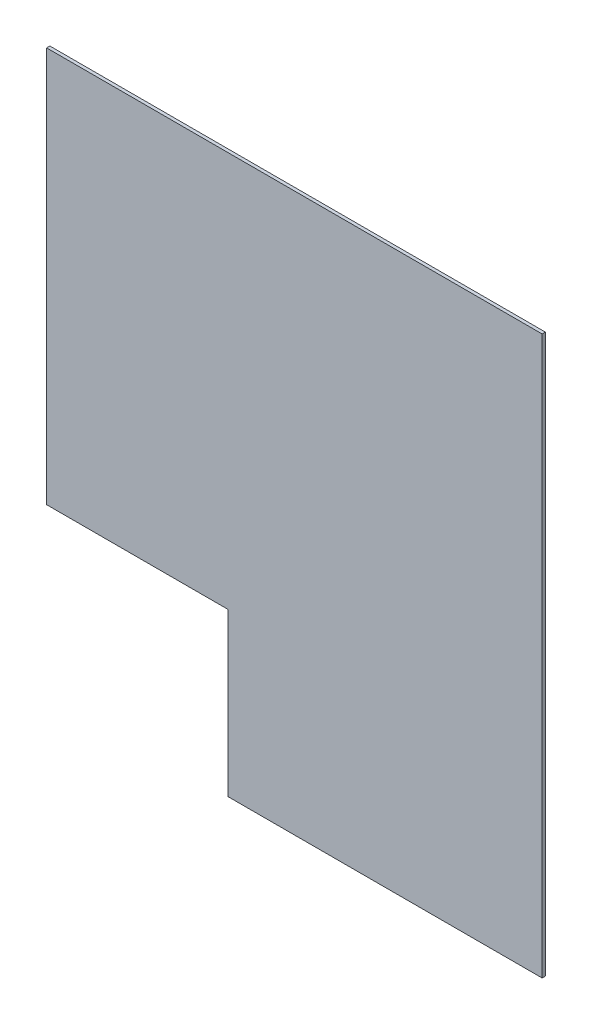
SolidWorks part; units mm, degrees
ref_plane "前视基准面" through (0, 0, 0) normal (0, 0, 1) x (1, 0, 0)
ref_plane "上视基准面" through (0, 0, 0) normal (0, 1, 0) x (1, 0, 0)
ref_plane "右视基准面" through (0, 0, 0) normal (1, 0, 0) x (0, 0, -1)
sketch "草图1" plane through (0, 0, 0) normal (0, 0, 1) x (1, 0, 0)
  line L1 (382, -430) -> (-382, -430)
  line L2 (382, -430) -> (382, 430)
  line L3 (382, 430) -> (-382, 430)
  line L4 (-382, -430) -> (-382, 430)
  line L5 (382, -430) -> (-382, 430) construction
  line L6 (382, 430) -> (-382, -430) construction
  point P0 (0, 0)
  dimension "D1" = 764
  dimension "D2" = 860
extrude "凸台-拉伸1" add sketch "草图1" along normal blind 5
sketch "草图2" plane through (0, 0, 5) normal (0, 0, 1) x (1, 0, 0)
  line L1 (-382, -430) -> (-102, -430)
  line L2 (-382, -430) -> (-382, -180)
  line L3 (-382, -180) -> (-102, -180)
  line L4 (-102, -430) -> (-102, -180)
  dimension "D1" = 280
  dimension "D2" = 250
extrude "切除-拉伸1" cut sketch "草图2" against normal up to next
